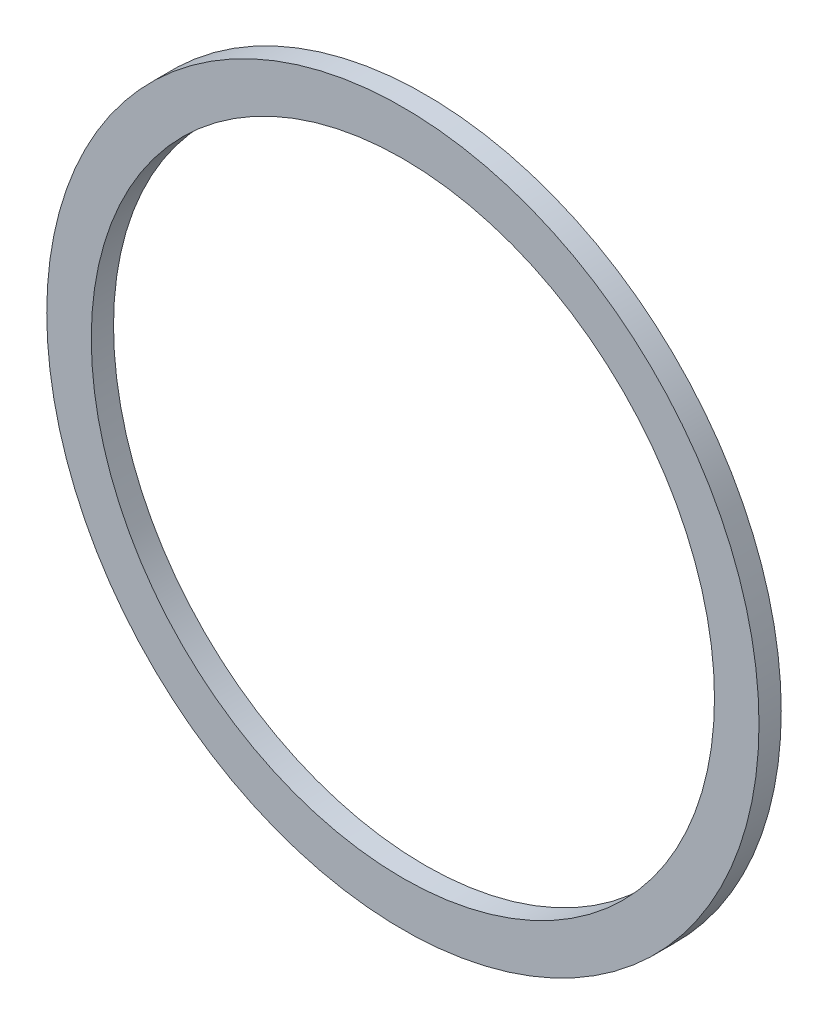
SolidWorks part; units mm, degrees
ref_plane "前视基准面" through (0, 0, 0) normal (0, 0, 1) x (1, 0, 0)
ref_plane "上视基准面" through (0, 0, 0) normal (0, 1, 0) x (1, 0, 0)
ref_plane "右视基准面" through (0, 0, 0) normal (1, 0, 0) x (0, 0, -1)
sketch "草图1" plane through (0, 0, 0) normal (0, 0, 1) x (1, 0, 0)
  circle A0 centre (0, 0) radius 40
  circle A1 centre (0, 0) radius 35
  dimension "D1" = 70
  dimension "D2" = 80
extrude "凸台-拉伸1" add sketch "草图1" along normal blind 2.5
